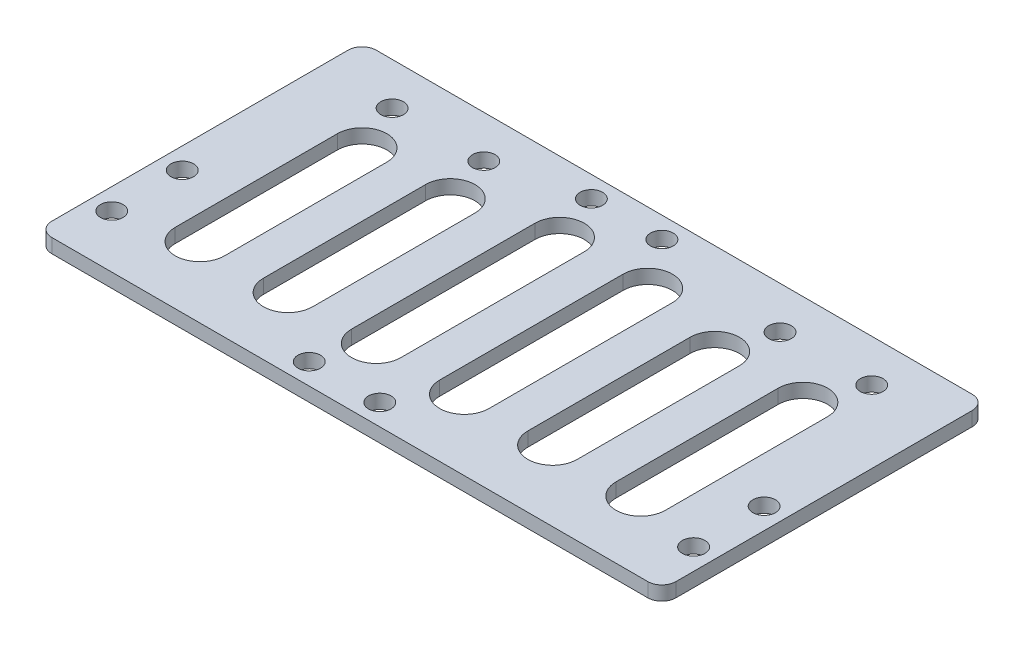
SolidWorks part; units mm, degrees
material "Thornel Mat VMA"
ref_plane "Front Plane" through (0, 0, 0) normal (0, 0, 1) x (1, 0, 0)
ref_plane "Top Plane" through (0, 0, 0) normal (0, 1, 0) x (1, 0, 0)
ref_plane "Right Plane" through (0, 0, 0) normal (1, 0, 0) x (0, 0, -1)
sketch "Sketch1" plane through (0, 0, 0) normal (0, 1, 0) x (1, 0, 0)
  line L0 (0, 23) -> (0, -23) construction
  line L1 (-44.25, 23) -> (44.25, 23)
  line L2 (-44.25, 23) -> (-44.25, -23)
  line L3 (-44.25, -23) -> (44.25, -23)
  line L4 (44.25, 23) -> (44.25, -23)
  line L5 (-44.25, 23) -> (44.25, -23) construction
  line L6 (-44.25, -23) -> (44.25, 23) construction
  line L7 (-41.25, -5.5) -> (-41.25, -15.5) construction
  line L8 (41.25, -5.5) -> (41.25, -15.5) construction
  line L9 (-8.75, -20) -> (1.25, -20) construction
  line L10 (-34, 17) -> (-21, 17) construction
  line L11 (21, 17) -> (34, 17) construction
  line L12 (-44.25, 0) -> (44.25, 0) construction
  line L13 (-8.75, 20) -> (1.25, 20) construction
  circle A0 centre (-41.25, -5.5) radius 1.6
  circle A1 centre (-41.25, -15.5) radius 1.6
  circle A4 centre (41.25, -15.5) radius 1.6
  circle A5 centre (41.25, -5.5) radius 1.6
  circle A6 centre (-8.75, -20) radius 1.6
  circle A7 centre (1.25, -20) radius 1.6
  circle A8 centre (-34, 17) radius 1.6
  circle A9 centre (-21, 17) radius 1.6
  circle A10 centre (21, 17) radius 1.6
  circle A11 centre (34, 17) radius 1.6
  circle A12 centre (1.25, 20) radius 1.6
  circle A13 centre (-8.75, 20) radius 1.6
  point P0 (0, 0)
  dimension "D1" = 3.2
  dimension "D7" = 3
  dimension "D9" = 13
  dimension "D11" = 3.2
  dimension "D2" = 3
  dimension "D3" = 7.5
  dimension "D4" = 10
  dimension "D5" = 46
  dimension "D6" = 88.5
  dimension "D8" = 35.5
  dimension "D10" = 6
  dimension "D12" = 42
extrude "Boss-Extrude1" add sketch "Sketch1" along normal blind 2
sketch "Sketch2" plane through (0, 2, 0) normal (0, 1, 0) x (1, 0, 0)
  line L0 (0, 23) -> (0, -23) construction
  line L1 (44.25, 23) -> (-44.25, 23) construction
  line L2 (-44.25, -23) -> (44.25, -23) construction
  line L3 (-44.25, -1.5) -> (44.25, -1.5) construction
  line L6 (-31.25, 10) -> (-31.25, -13) construction
  line L7 (-27.75, 10) -> (-27.75, -13)
  line L8 (-34.75, 10) -> (-34.75, -13)
  line L9 (-18.75, 10) -> (-18.75, -13) construction
  line L10 (-15.25, 10) -> (-15.25, -13)
  line L11 (-22.25, 10) -> (-22.25, -13)
  line L12 (-6.25, 13) -> (-6.25, -13) construction
  line L13 (-2.75, 13) -> (-2.75, -13)
  line L14 (-9.75, 13) -> (-9.75, -13)
  line L15 (6.25, 13) -> (6.25, -13) construction
  line L16 (9.75, 13) -> (9.75, -13)
  line L17 (2.75, 13) -> (2.75, -13)
  line L18 (18.75, 10) -> (18.75, -13) construction
  line L19 (22.25, 10) -> (22.25, -13)
  line L20 (15.25, 10) -> (15.25, -13)
  line L21 (31.25, 10) -> (31.25, -13) construction
  line L22 (34.75, 10) -> (34.75, -13)
  line L23 (27.75, 10) -> (27.75, -13)
  line L24 (44.25, -23) -> (44.25, 23) construction
  line L27 (-44.25, 23) -> (-44.25, -23) construction
  arc A0 (-27.75, 10) -> (-34.75, 10) centre (-31.25, 10) ccw
  arc A1 (-34.75, -13) -> (-27.75, -13) centre (-31.25, -13) ccw
  arc A2 (-15.25, 10) -> (-22.25, 10) centre (-18.75, 10) ccw
  arc A3 (-22.25, -13) -> (-15.25, -13) centre (-18.75, -13) ccw
  arc A4 (-2.75, 13) -> (-9.75, 13) centre (-6.25, 13) ccw
  arc A5 (-9.75, -13) -> (-2.75, -13) centre (-6.25, -13) ccw
  arc A6 (9.75, 13) -> (2.75, 13) centre (6.25, 13) ccw
  arc A7 (2.75, -13) -> (9.75, -13) centre (6.25, -13) ccw
  arc A8 (22.25, 10) -> (15.25, 10) centre (18.75, 10) ccw
  arc A9 (15.25, -13) -> (22.25, -13) centre (18.75, -13) ccw
  arc A10 (34.75, 10) -> (27.75, 10) centre (31.25, 10) ccw
  arc A11 (27.75, -13) -> (34.75, -13) centre (31.25, -13) ccw
  circle A14 centre (-8.75, -20) radius 1.6 construction
  circle A15 centre (-8.75, 20) radius 1.6 construction
  point P14 (-31.25, -1.5)
  point P22 (-18.75, -1.5)
  point P29 (-6.25, 0)
  point P36 (6.25, 0)
  point P43 (18.75, -1.5)
  point P50 (31.25, -1.5)
  dimension "D1" = 3.5
  dimension "D2" = 23
  dimension "D4" = 12.5
  dimension "D5" = 7
  dimension "D3" = 7
extrude "Cut-Extrude1" cut sketch "Sketch2" against normal through all
fillet "Fillet1" radius 2 4 edges at (44.25, 1, -23) (44.25, 1, 23) (-44.25, 1, 23) (-44.25, 1, -23)
